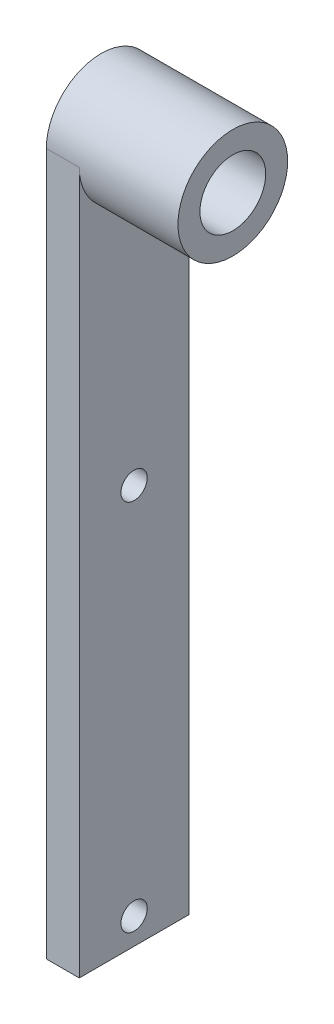
SolidWorks part; units mm, degrees
ref_plane "前视基准面" through (0, 0, 0) normal (0, 0, 1) x (1, 0, 0)
ref_plane "上视基准面" through (0, 0, 0) normal (0, 1, 0) x (1, 0, 0)
ref_plane "右视基准面" through (0, 0, 0) normal (1, 0, 0) x (0, 0, -1)
sketch "草图1" plane through (0, 0, 0) normal (1, 0, 0) x (0, 0, -1)
  line L1 (-25, 160) -> (25, 160)
  line L2 (-25, 160) -> (-25, -160)
  line L3 (-25, -160) -> (25, -160)
  line L4 (25, 160) -> (25, -160)
  line L5 (-25, 160) -> (25, -160) construction
  line L6 (-25, -160) -> (25, 160) construction
  point P0 (0, 0)
  dimension "D1" = 50
  dimension "D2" = 320
extrude "凸台-拉伸1" add sketch "草图1" along normal mid plane 15
sketch "草图2" plane through (0, 0, 0) normal (1, 0, 0) x (0, 0, -1)
  line L0 (25, 160) -> (-25, 160) construction
  circle A0 centre (0, 160) radius 25
  dimension "D1" = 50
extrude "凸台-拉伸2" add sketch "草图2" along normal blind 52.5 and the other way blind 7.5
sketch "草图3" plane through (52.5, 0, 0) normal (1, 0, 0) x (0, 0, -1)
  circle A0 centre (0, 160) radius 15
  dimension "D1" = 30
extrude "切除-拉伸1" cut sketch "草图3" against normal through all
hole_wizard "Ø12.0 (12) 直径孔1" positions "草图4" profile "草图5" hole size "Ø12.0" standard "ISO" end condition through all
sketch "草图4" plane through (-7.5, 0, 0) normal (-1, 0, 0) x (0, 0, 1)
  line L0 (25, -160) -> (-25, -160) construction
  point P0 (0, 22)
  point P2 (0, -148)
  dimension "D1" = 12
  dimension "D2" = 170
sketch "草图5" plane through (-7.5, 22, 0) normal (0, 1, 0) x (0, 0, 1)
  line L0 (0, 0) -> (0, 60)
  line L1 (0, 60) -> (6, 60)
  line L2 (6, 60) -> (6, 0)
  line L5 (6, 0) -> (0, 0)
  line L11 (0, -6.35) -> (0, 107.95) construction
  dimension "通孔孔直径" = 12
  dimension "通孔孔深度" = 60
